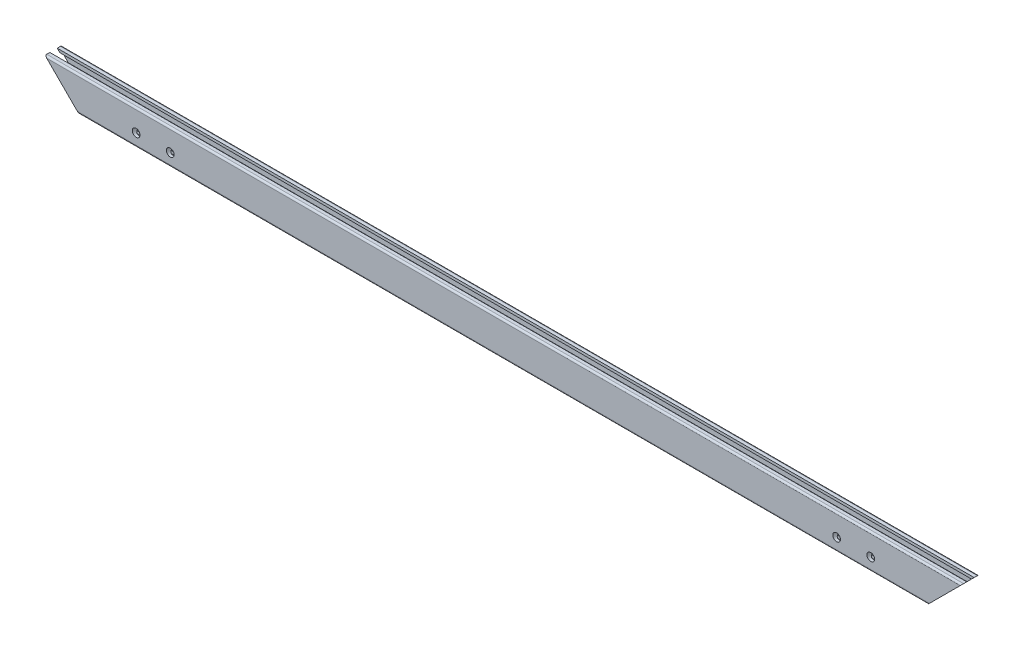
SolidWorks part; units mm, degrees
ref_plane "前视" through (0, 0, 0) normal (0, 0, 1) x (1, 0, 0)
ref_plane "上视" through (0, 0, 0) normal (0, 1, 0) x (1, 0, 0)
ref_plane "右视" through (0, 0, 0) normal (1, 0, 0) x (0, 0, -1)
sketch3d "3D草图1"
  line L0 (-402.5, 0, 0) -> (402.5, 0, 0)
  dimension "D1" = 805
other "结构构件1"
ref_plane "基准面1" through (-402.5, 0, 0) normal (1, 0, 0) x (0, 0, -1)
sketch "Sketch11" plane through (-402.5, 0, 0) normal (1, 0, 0) x (0, 0, -1)
  line L1 (0, 16.311) -> (0, -16.311) construction
  line L2 (0, 0) -> (9.513, 0) construction
  line L3 (-6, -15) -> (-3.25, -15)
  line L4 (-7.5, -13.5) -> (-7.5, 13.5)
  line L5 (-6, 15) -> (-3.25, 15)
  line L6 (7.5, -13.5) -> (7.5, 13.5)
  line L17 (3.25, 15) -> (6, 15)
  line L20 (-5, 12.7) -> (-5, 7)
  line L21 (-3.25, 12.7) -> (-5, 12.7)
  line L24 (5, 12.7) -> (5, 7)
  line L25 (3.25, 12.7) -> (5, 12.7)
  line L26 (-3.25, 15) -> (-3.25, 12.7)
  line L27 (3.25, 15) -> (3.25, 12.7)
  line L40 (5, -12.7) -> (5, -7)
  line L41 (3.25, -12.7) -> (5, -12.7)
  line L44 (-5, -12.7) -> (-5, -7)
  line L45 (-3.25, -12.7) -> (-5, -12.7)
  line L47 (3.25, -15) -> (3.25, -12.7)
  line L48 (-3.25, -15) -> (-3.25, -12.7)
  line L49 (3.25, -15) -> (6, -15)
  arc A0 (-6, -15) -> (-7.5, -13.5) centre (-6, -13.5) cw
  arc A1 (6, -15) -> (7.5, -13.5) centre (6, -13.5) ccw
  arc A2 (6, 15) -> (7.5, 13.5) centre (6, 13.5) cw
  arc A3 (-7.5, 13.5) -> (-6, 15) centre (-6, 13.5) cw
  circle A4 centre (0, 0) radius 2.5
  arc A5 (-5, 7) -> (5, 7) centre (0, 10.3166) ccw
  arc A6 (-5, -7) -> (5, -7) centre (0, -10.3166) cw
  point P4 (0, 0)
  point P21 (0, 0)
  point P44 (-7.5, 15)
  point P45 (7.5, 15)
  point P46 (7.5, -15)
  point P47 (-7.5, -15)
  point P48 (0, -15)
  point P49 (0, 15)
  dimension "D1" = 30
  dimension "D2" = 15
  dimension "D3" = 1.5
  dimension "D4" = 5
  dimension "D5" = 6.5
  dimension "D6" = 6
  dimension "D7" = 8
  dimension "D8" = 10
  dimension "D9" = 2.3
sketch "草图4" plane through (0, 0, 7.5) normal (0, 0, 1) x (1, 0, 0)
  line L0 (-402.5, 15) -> (-372.5, -15)
  line L1 (402.5, -15) -> (-402.5, -15) construction
  line L2 (0, 0) -> (0, -85.0329) construction
  line L3 (-372.5, -15) -> (-402.5, -15)
  line L4 (-402.5, -15) -> (-402.5, 15)
  line L5 (402.5, -15) -> (402.5, 15)
  line L6 (372.5, -15) -> (402.5, -15)
  line L7 (402.5, 15) -> (372.5, -15)
extrude "切除-拉伸1" cut sketch "草图4" against normal through all
hole_wizard "M8 螺纹孔1" positions "草图6" profile "草图7" tap size "M8" standard "Iso" end condition through all
sketch "草图6" plane through (0, 0, 7.5) normal (0, 0, 1) x (1, 0, 0)
  line L0 (0, 0) -> (0, -60.6345) construction
  line L2 (402.5, 15) -> (-402.5, 15) construction
  point P0 (-322.5, -4)
  point P2 (-292.5, -4)
  point P9 (292.5, -4)
  point P10 (322.5, -4)
  dimension "D1" = 30
  dimension "D2" = 19
  dimension "D3" = 80
sketch "草图7" plane through (-322.5, -4, 7.5) normal (1, 0, 0) x (0, -1, 0)
  line L0 (0, 0) -> (0, 15)
  line L1 (0, 15) -> (3.4, 15)
  line L2 (3.4, 15) -> (3.4, 0)
  line L5 (3.4, 0) -> (0, 0)
  line L11 (0, -6.35) -> (0, 107.95) construction
  dimension "通孔螺纹孔钻头直径" = 6.8
  dimension "通孔螺纹孔钻头深度" = 15
cosmetic thread "孔螺蚊线1" parameters "D2"=8
cosmetic thread "孔螺蚊线2" parameters "D2"=8
cosmetic thread "孔螺蚊线3" parameters "D2"=8
cosmetic thread "孔螺蚊线4" parameters "D2"=8
